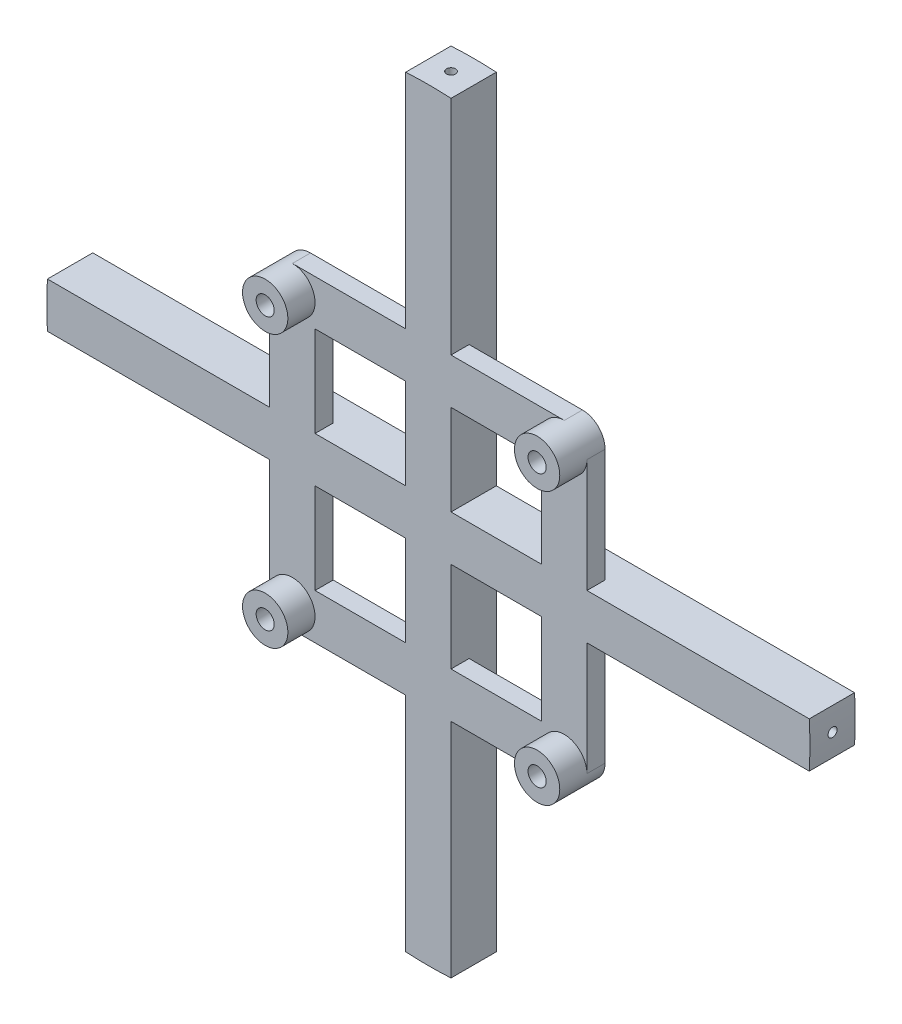
from build123d import *

# Parameters (mm, degrees)
BOSS_EXTRUDE1_DEPTH     = 5
BOSS_EXTRUDE2_DEPTH     = 2
BOSS_EXTRUDE2_2_DEPTH   = 2
BOSS_EXTRUDE2_3_DEPTH   = 2
BOSS_EXTRUDE2_4_DEPTH   = 2
SKETCH3_R               = 1
CUT_EXTRUDE1_DEPTH      = 60.747970677
SKETCH5_R               = 2.5
SKETCH5_R_2             = 1
BOSS_EXTRUDE3_DEPTH     = 3
CUT_EXTRUDE2_DEPTH      = 60.747970677
SKETCH12_R              = 2.5
BOSS_EXTRUDE4_DEPTH     = 3
SKETCH13_R              = 1
CUT_EXTRUDE3_DEPTH      = 61.073455036
CUT_EXTRUDE4_DEPTH      = 60.747970677
CUT_EXTRUDE5_DEPTH      = 61.073455036
CUT_EXTRUDE5_DEPTH_BACK = 61.073455036
SKETCH17_R              = 0.5
CUT_EXTRUDE6_DEPTH      = 61.073455106
CUT_EXTRUDE6_DEPTH_BACK = 61.073455106
SKETCH18_R              = 0.5


with BuildPart() as part:
    # Sketch1 → Boss-Extrude1 (new body)
    with BuildSketch(Plane.XY):
        with BuildLine():
            Line((-42.025706419, 2.5), (-2.5, 2.5))
            Line((-2.5, 2.5), (-2.5, 42.025706419))
            ThreePointArc((-2.5, 42.025706419), (0, 42.1), (2.5, 42.025706419))
            Line((2.5, 42.025706419), (2.5, 2.5))
            Line((2.5, 2.5), (42.025706419, 2.5))
            ThreePointArc((42.025706419, 2.5), (42.1, 0), (42.025706419, -2.5))
            Line((42.025706419, -2.5), (2.5, -2.5))
            Line((2.5, -2.5), (2.5, -42.025706419))
            ThreePointArc((2.5, -42.025706419), (0, -42.1), (-2.5, -42.025706419))
            Line((-2.5, -42.025706419), (-2.5, -2.5))
            Line((-2.5, -2.5), (-42.025706419, -2.5))
            ThreePointArc((-42.025706419, -2.5), (-42.1, 0), (-42.025706419, 2.5))
        make_face()
    extrude(amount=BOSS_EXTRUDE1_DEPTH)



with BuildPart() as body_2:
    # Sketch2 → Boss-Extrude2 (new body)
    with BuildSketch(Plane.XY.offset(5)):
        Polygon((2.5, 12.5), (12.5, 12.5), (12.5, 2.5), (17.5, 2.5), (17.5, 17.5), (2.5, 17.5), align=None)
    extrude(amount=-BOSS_EXTRUDE2_DEPTH)

    # Sketch3 → Cut-Extrude1 (cut, through all)
    with BuildSketch(Plane.XY.offset(5)):
        with Locations((15, 15)):
            Circle(SKETCH3_R)
    extrude(amount=-CUT_EXTRUDE1_DEPTH, mode=Mode.SUBTRACT)


with BuildPart() as body_3:
    # Sketch2 → Boss-Extrude2 2 (new body)
    with BuildSketch(Plane.XY.offset(5)):
        Polygon((-12.5, 12.5), (-2.5, 12.5), (-2.5, 17.5), (-17.5, 17.5), (-17.5, 2.5), (-12.5, 2.5), align=None)
    extrude(amount=-BOSS_EXTRUDE2_2_DEPTH)



with BuildPart() as body_4:
    # Sketch2 → Boss-Extrude2 3 (new body)
    with BuildSketch(Plane.XY.offset(5)):
        Polygon((-12.5, -12.5), (-2.5, -12.5), (-2.5, -17.5), (-17.5, -17.5), (-17.5, -2.5), (-12.5, -2.5), align=None)
    extrude(amount=-BOSS_EXTRUDE2_3_DEPTH)


with BuildPart() as body_5:
    # Sketch2 → Boss-Extrude2 4 (new body)
    with BuildSketch(Plane.XY.offset(5)):
        Polygon((12.5, -2.5), (12.5, -12.5), (2.5, -12.5), (2.5, -17.5), (17.5, -17.5), (17.5, -2.5), align=None)
    extrude(amount=-BOSS_EXTRUDE2_4_DEPTH)


with BuildPart() as part_1:
    add(part.part)

    add(body_2.part)  # Boss-Extrude3 merges body 2
    # Sketch5 → Boss-Extrude3 (add)
    with BuildSketch(Plane.XY.offset(5)):
        with Locations((15, 15)):
            Circle(SKETCH5_R)
        with Locations((15, 15)):
            Circle(SKETCH5_R_2, mode=Mode.SUBTRACT)
    extrude(amount=BOSS_EXTRUDE3_DEPTH)

    # Sketch6 → Cut-Extrude2 (cut, through all)
    with BuildSketch(Plane.XY.offset(5)):
        with BuildLine():
            ThreePointArc((17.5, 15), (16.767766953, 16.767766953), (15, 17.5))
            Line((15, 17.5), (17.5, 17.5))
            Line((17.5, 17.5), (17.5, 15))
        make_face()
    extrude(amount=-CUT_EXTRUDE2_DEPTH, mode=Mode.SUBTRACT)


with BuildPart() as body_3_1:
    add(body_3.part)

    add(part_1.part)  # Boss-Extrude4 merges part

    add(body_5.part)  # Boss-Extrude4 merges body 5

    add(body_4.part)  # Boss-Extrude4 merges body 4
    # Sketch12 → Boss-Extrude4 (add)
    with BuildSketch(Plane.XY.offset(5)):
        with Locations((15, -15)):
            Circle(SKETCH12_R)
        with Locations(Location((-15, -15, 0), (0, 0, 180))):
            Circle(SKETCH12_R)
        with Locations(Location((-15, 15, 0), (0, 0, 180))):
            Circle(SKETCH12_R)
    extrude(amount=BOSS_EXTRUDE4_DEPTH)

    # Sketch13 → Cut-Extrude3 (cut, through all)
    with BuildSketch(Plane.XY.offset(8)):
        with Locations((15, -15)):
            Circle(SKETCH13_R)
        with Locations((-15, -15)):
            Circle(SKETCH13_R)
        with Locations((-15, 15)):
            Circle(SKETCH13_R)
    extrude(amount=-CUT_EXTRUDE3_DEPTH, mode=Mode.SUBTRACT)

    # Sketch14 → Cut-Extrude4 (cut, through all)
    with BuildSketch(Plane.XY.offset(5)):
        with BuildLine():
            Line((-15, 17.5), (-17.5, 17.5))
            Line((-17.5, 17.5), (-17.5, 15))
            ThreePointArc((-17.5, 15), (-16.767766953, 16.767766953), (-15, 17.5))
        make_face()
        with BuildLine():
            Line((-17.5, -15), (-17.5, -17.5))
            Line((-17.5, -17.5), (-15, -17.5))
            ThreePointArc((-15, -17.5), (-16.767766953, -16.767766953), (-17.5, -15))
        make_face()
        with BuildLine():
            Line((15, -17.5), (17.5, -17.5))
            Line((17.5, -17.5), (17.5, -15))
            ThreePointArc((17.5, -15), (16.767766953, -16.767766953), (15, -17.5))
        make_face()
    extrude(amount=-CUT_EXTRUDE4_DEPTH, mode=Mode.SUBTRACT)

    # Sketch17 → Cut-Extrude5 (cut, two sides: drawn at the far end of the back side and taken through both)
    with BuildSketch(Plane(origin=(0, 0, 0), x_dir=(1, 0, 0), z_dir=(0, 1, 0)).offset(-CUT_EXTRUDE5_DEPTH_BACK)):
        with Locations(Location((0, -2.5, 0), (0, 0, 270))):
            Circle(SKETCH17_R)
    extrude(amount=CUT_EXTRUDE5_DEPTH + CUT_EXTRUDE5_DEPTH_BACK, mode=Mode.SUBTRACT)

    # Sketch18 → Cut-Extrude6 (cut, two sides: drawn at the far end of the back side and taken through both)
    with BuildSketch(Plane(origin=(0, 0, 0), x_dir=(0, 0, -1), z_dir=(1, 0, 0)).offset(-CUT_EXTRUDE6_DEPTH_BACK)):
        with Locations((-2.5, 0)):
            Circle(SKETCH18_R)
    extrude(amount=CUT_EXTRUDE6_DEPTH + CUT_EXTRUDE6_DEPTH_BACK, mode=Mode.SUBTRACT)


solid = body_3_1.part
